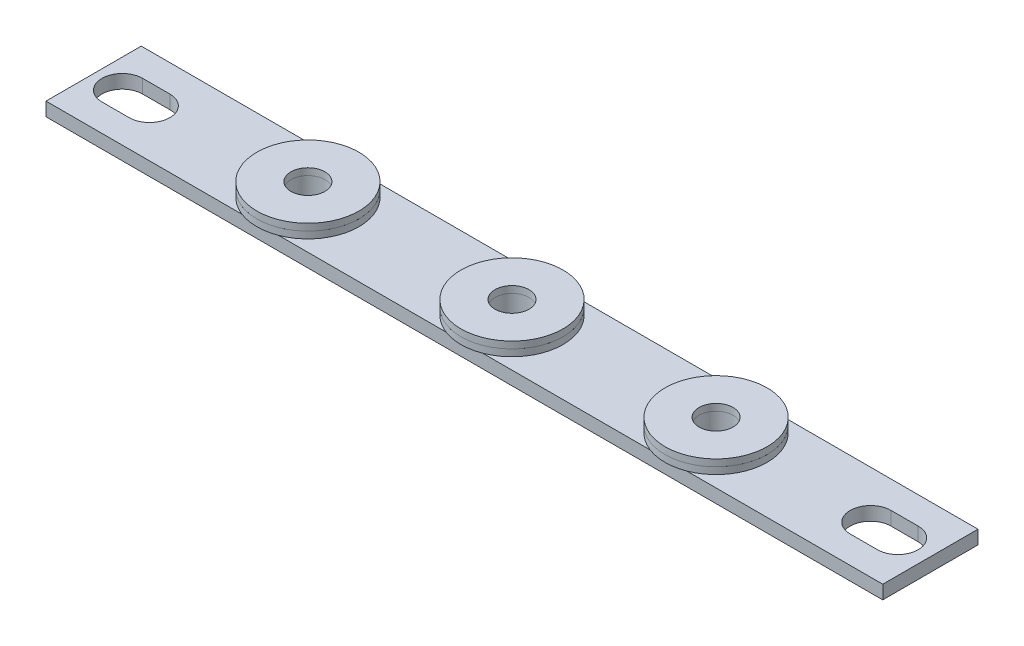
from build123d import *

# Parameters (mm, degrees)
SKETCH_1_W        = 123
SKETCH_1_H        = 14
SKETCH_1_R        = 2.5
EXTRUDE_1_DEPTH   = 2
SKETCH_2_R        = 7.5
SKETCH_2_R_2      = 2.5
EXTRUDE_2_DEPTH   = 1
SKETCH_3_R        = 7.5
SKETCH_3_R_2      = 2.5
EXTRUDE_3_DEPTH   = 1
EXTRUDE_3_2_DEPTH = 1
EXTRUDE_3_3_DEPTH = 1


with BuildPart() as part:
    # 草图1 → 凸台-拉伸1 (new body)
    with BuildSketch(Plane(origin=(0, 0, 0), x_dir=(1, 0, 0), z_dir=(0, 1, 0))):
        Rectangle(SKETCH_1_W, SKETCH_1_H)
        with Locations(Location((-30, 0, 0), (0, 0, 270))):
            Circle(SKETCH_1_R, mode=Mode.SUBTRACT)
        with Locations(Location((0, 0, 0), (0, 0, 270))):
            Circle(SKETCH_1_R, mode=Mode.SUBTRACT)
        with Locations(Location((30, 0, 0), (0, 0, 270))):
            Circle(SKETCH_1_R, mode=Mode.SUBTRACT)
        with BuildLine():
            Line((-57.285714286, 3), (-53.285714286, 3))
            ThreePointArc((-53.285714286, 3), (-50.285714286, 0), (-53.285714286, -3))
            Line((-53.285714286, -3), (-57.285714286, -3))
            ThreePointArc((-57.285714286, -3), (-60.285714286, 0), (-57.285714286, 3))
        make_face(mode=Mode.SUBTRACT)
        with BuildLine():
            Line((52.714285714, 3), (56.714285714, 3))
            ThreePointArc((56.714285714, 3), (59.714285714, 0), (56.714285714, -3))
            Line((56.714285714, -3), (52.714285714, -3))
            ThreePointArc((52.714285714, -3), (49.714285714, 0), (52.714285714, 3))
        make_face(mode=Mode.SUBTRACT)
    extrude(amount=EXTRUDE_1_DEPTH)

    # 草图2 → 凸台-拉伸2 (add)
    # profile 1 of 3: a face of its own
    with BuildSketch(Plane(origin=(0, 2, 0), x_dir=(1, 0, 0), z_dir=(0, 1, 0))):
        with Locations(Location((-30, 0, 0), (0, 0, 68.960530219))):
            Circle(SKETCH_2_R)
        with Locations(Location((-30, 0, 0), (0, 0, 270))):
            Circle(SKETCH_2_R_2, mode=Mode.SUBTRACT)
    # profile 2 of 3: a face of its own
    with BuildSketch(Plane(origin=(0, 2, 0), x_dir=(1, 0, 0), z_dir=(0, 1, 0))):
        with Locations(Location((0, 0, 0), (0, 0, 111.039469781))):
            Circle(SKETCH_2_R)
        with Locations(Location((0, 0, 0), (0, 0, 270))):
            Circle(SKETCH_2_R_2, mode=Mode.SUBTRACT)
    # profile 3 of 3: a face of its own
    with BuildSketch(Plane(origin=(0, 2, 0), x_dir=(1, 0, 0), z_dir=(0, 1, 0))):
        with Locations(Location((30, 0, 0), (0, 0, 68.960530219))):
            Circle(SKETCH_2_R)
        with Locations(Location((30, 0, 0), (0, 0, 270))):
            Circle(SKETCH_2_R_2, mode=Mode.SUBTRACT)
    extrude(amount=EXTRUDE_2_DEPTH)


with BuildPart() as body_2:
    # 草图3 → 凸台-拉伸3 (new body)
    with BuildSketch(Plane(origin=(0, 3, 0), x_dir=(1, 0, 0), z_dir=(0, 1, 0))):
        with Locations(Location((-30, 0, 0), (0, 0, 270))):
            Circle(SKETCH_3_R)
        with Locations(Location((-30, 0, 0), (0, 0, 270))):
            Circle(SKETCH_3_R_2, mode=Mode.SUBTRACT)
    extrude(amount=EXTRUDE_3_DEPTH)


with BuildPart() as body_3:
    # 草图3 → Extrude 3 2 (new body)
    with BuildSketch(Plane(origin=(0, 3, 0), x_dir=(1, 0, 0), z_dir=(0, 1, 0))):
        with Locations(Location((0, 0, 0), (0, 0, 270))):
            Circle(SKETCH_3_R)
        with Locations(Location((0, 0, 0), (0, 0, 270))):
            Circle(SKETCH_3_R_2, mode=Mode.SUBTRACT)
    extrude(amount=EXTRUDE_3_2_DEPTH)


with BuildPart() as body_4:
    # 草图3 → Extrude 3 3 (new body)
    with BuildSketch(Plane(origin=(0, 3, 0), x_dir=(1, 0, 0), z_dir=(0, 1, 0))):
        with Locations(Location((30, 0, 0), (0, 0, 270))):
            Circle(SKETCH_3_R)
        with Locations(Location((30, 0, 0), (0, 0, 270))):
            Circle(SKETCH_3_R_2, mode=Mode.SUBTRACT)
    extrude(amount=EXTRUDE_3_3_DEPTH)


solid = Compound([part.part, body_2.part, body_3.part, body_4.part])
